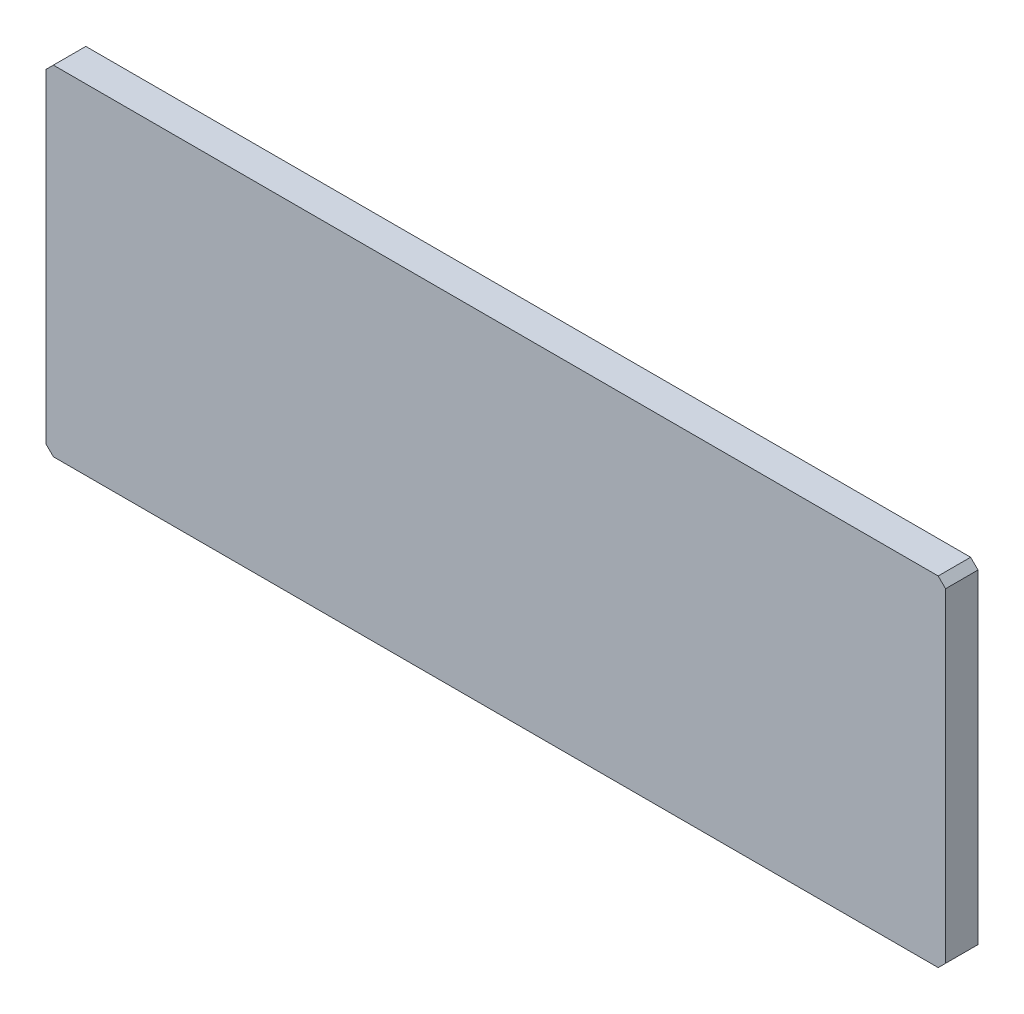
from build123d import *

# Parameters (mm, degrees)
SKETCH1_W           = 610
SKETCH1_H           = 230
BOSS_EXTRUDE1_DEPTH = 22
CHAMFER1_SIZE       = 5


with BuildPart() as part:
    # Sketch1 → Boss-Extrude1 (new body)
    with BuildSketch(Plane.XY):
        with Locations((258.381462009, 97.028215789)):
            Rectangle(SKETCH1_W, SKETCH1_H)
    extrude(amount=BOSS_EXTRUDE1_DEPTH)

    # Chamfer1
    chamfer1_edges = [part.edges().sort_by_distance(p)[0] for p in [
        (563.381462009, 212.028215789, 11),
        (563.381462009, -17.971784211, 11),
        (-46.618537991, -17.971784211, 11),
        (-46.618537991, 212.028215789, 11),
    ]]
    chamfer(chamfer1_edges, length=CHAMFER1_SIZE)


solid = part.part
